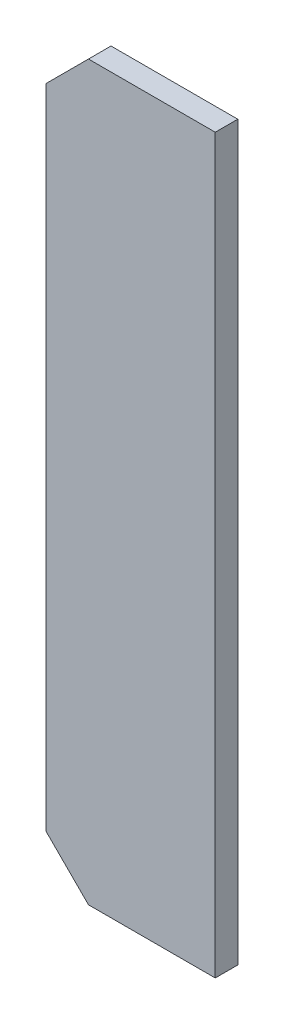
from build123d import *

# Parameters (mm, degrees)
SKETCH1_W           = 60
SKETCH1_H           = 260
BOSS_EXTRUDE1_DEPTH = 8
CHAMFER1_SIZE       = 15


with BuildPart() as part:
    # Sketch1 → Boss-Extrude1 (new body)
    with BuildSketch(Plane.XY):
        Rectangle(SKETCH1_W, SKETCH1_H)
    extrude(amount=BOSS_EXTRUDE1_DEPTH)

    # Chamfer1
    chamfer1_edges = [part.edges().sort_by_distance(p)[0] for p in [
        (-30, 130, 4),
        (-30, -130, 4),
    ]]
    chamfer(chamfer1_edges, length=CHAMFER1_SIZE)


solid = part.part
